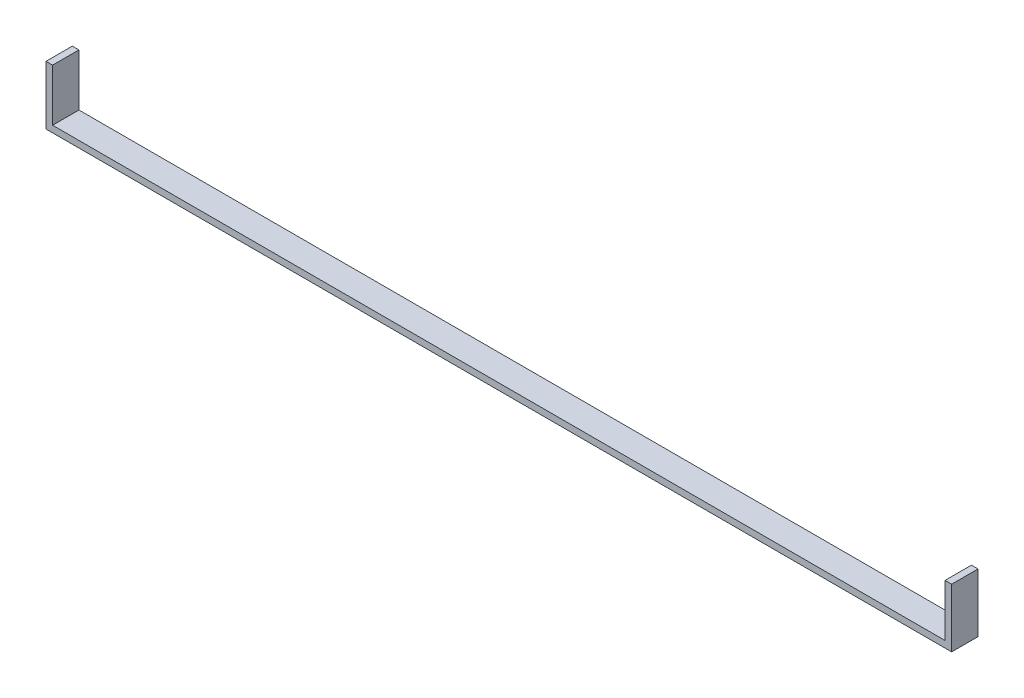
from build123d import *

# Parameters (mm, degrees)
SKETCH_1_W      = 1354
SKETCH_1_H      = 40
EXTRUDE_1_DEPTH = 10
SKETCH_2_W      = 40
SKETCH_2_H      = 89
EXTRUDE_2_DEPTH = 10


with BuildPart() as part:
    # 草图1 → 凸台-拉伸1 (new body)
    with BuildSketch(Plane(origin=(0, 0, 0), x_dir=(1, 0, 0), z_dir=(0, 1, 0))):
        Rectangle(SKETCH_1_W, SKETCH_1_H)
    extrude(amount=EXTRUDE_1_DEPTH)

    # 草图2 → 凸台-拉伸2 (add)
    with BuildSketch(Plane.ZY.offset(677)):
        with Locations((0, 44.5)):
            Rectangle(SKETCH_2_W, SKETCH_2_H)
    extrude_2 = extrude(amount=EXTRUDE_2_DEPTH)

    # 镜向1: 凸台-拉伸2 across plane
    add(extrude_2.mirror(Plane(origin=(0, 0, 0), x_dir=(0, 0, 1), z_dir=(1, 0, 0))))


solid = part.part
